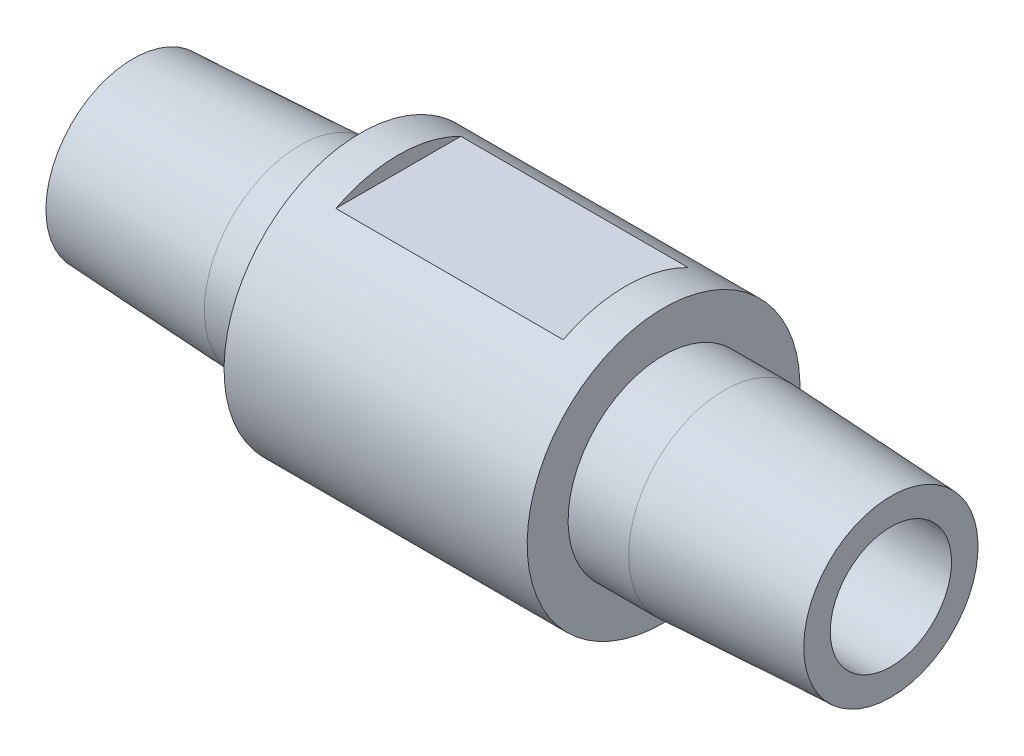
from build123d import *

# Parameters (mm, degrees)
SKETCH_2_OUTSIDE_W   = 31.222
SKETCH_2_OUTSIDE_H   = 31.222
SKETCH_2_OUTSIDE_W_2 = 20.905852418
SKETCH_2_OUTSIDE_H_2 = 16
CUT_EXTRUDE_1_DEPTH  = 7.5


with BuildPart() as part:
    # 草图1 → 旋转1 (revolve)
    with BuildSketch(Plane.XY, mode=Mode.PRIVATE) as revolve_1_sk:
        Polygon((0, 4), (0, 5.75), (11, 6.3), (15, 6.3), (15, 9), (35, 9), (35, 6.3), (39, 6.3), (50, 5.75), (50, 4), align=None)
    revolve(revolve_1_sk.sketch.rotate(Axis((0, 0, 0), (1, 0, 0)), 180), axis=Axis((0, 0, 0), (1, 0, 0)))

    # 草图2 outside → 切除-拉伸1 (cut, symmetric)
    with BuildSketch(Plane.ZY.offset(-25)):
        Rectangle(SKETCH_2_OUTSIDE_W, SKETCH_2_OUTSIDE_H)
        Rectangle(SKETCH_2_OUTSIDE_W_2, SKETCH_2_OUTSIDE_H_2, mode=Mode.SUBTRACT)
    extrude(amount=CUT_EXTRUDE_1_DEPTH, both=True, mode=Mode.SUBTRACT)


solid = part.part
